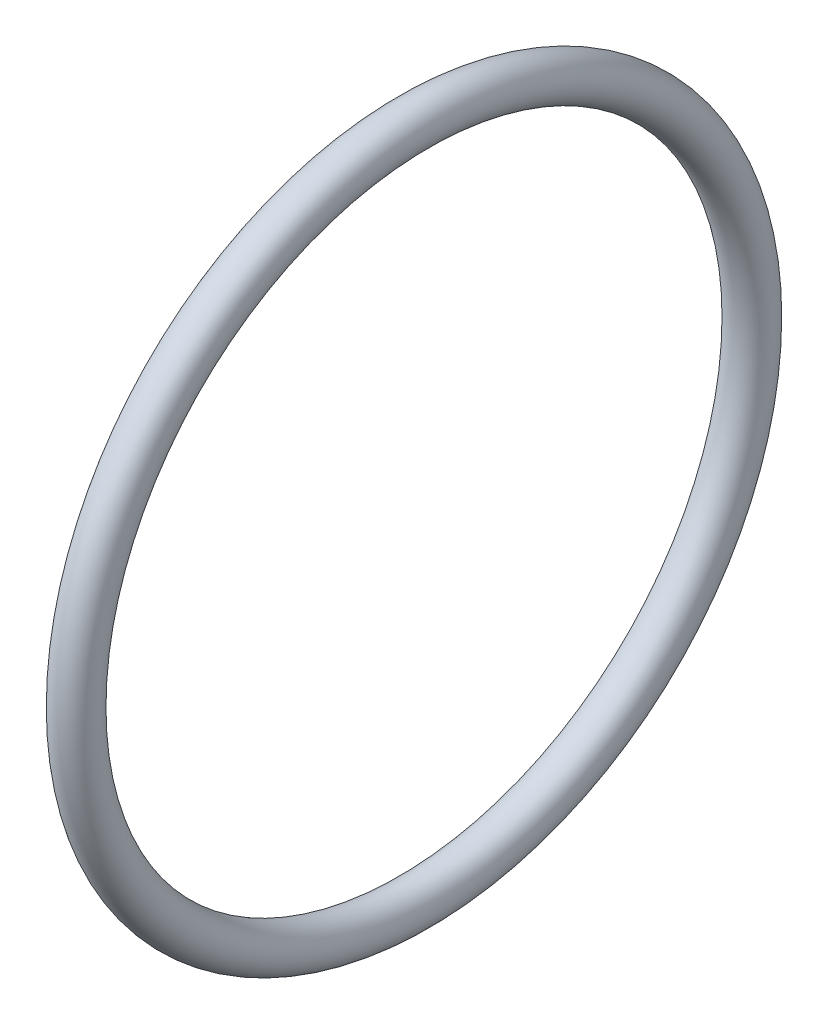
from build123d import *

# Parameters (mm, degrees)
SKETCH_1_R = 2.5


with BuildPart() as part:
    # 草图1 → 旋转1 (revolve)
    with BuildSketch(Plane.XY, mode=Mode.PRIVATE) as revolve_1_sk:
        with Locations((0, 40)):
            Circle(SKETCH_1_R)
    revolve(revolve_1_sk.sketch.rotate(Axis((-21.92893401, 0, 0), (1, 0, 0)), 90), axis=Axis((-21.92893401, 0, 0), (1, 0, 0)))


solid = part.part
